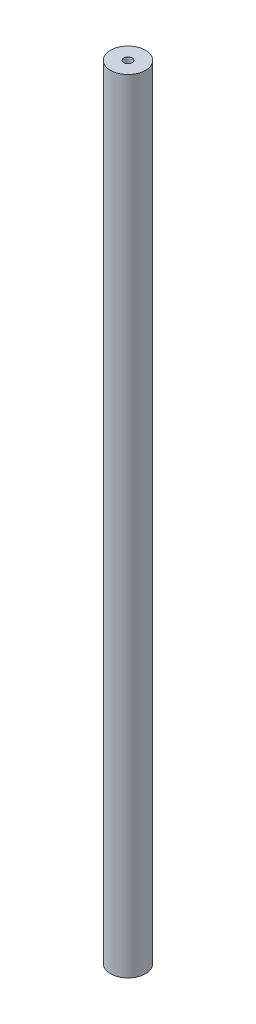
from build123d import *

# Parameters (mm, degrees)
SKETCH1_W = 0.8
SKETCH1_H = 47


with BuildPart() as part:
    # Sketch1 → Revolve1 (revolve)
    with BuildSketch(Plane.XY, mode=Mode.PRIVATE) as revolve1_sk:
        with Locations((-0.65, 23.5)):
            Rectangle(SKETCH1_W, SKETCH1_H)
    revolve(revolve1_sk.sketch.rotate(Axis((0, -3.568356633, 0), (0, 1, 0)), 270), axis=Axis((0, -3.568356633, 0), (0, 1, 0)))


solid = part.part
